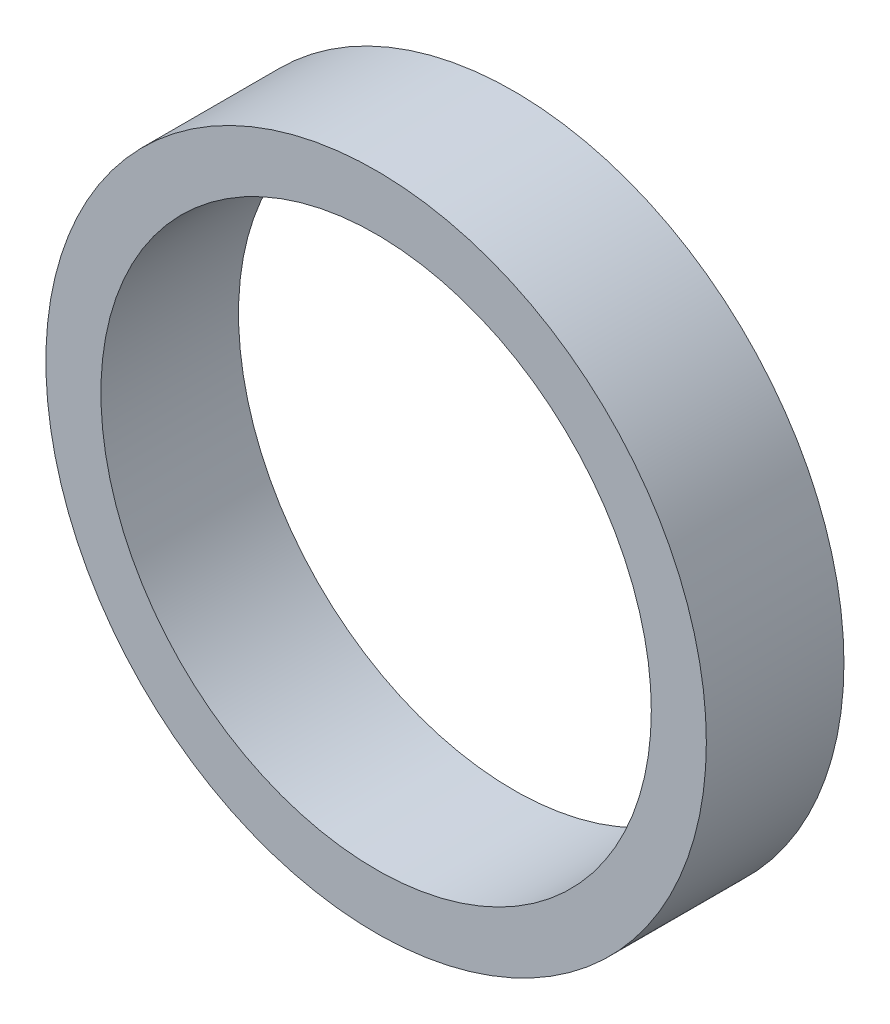
SolidWorks part; units mm, degrees
ref_plane "前视基准面" through (0, 0, 0) normal (0, 0, 1) x (1, 0, 0)
ref_plane "上视基准面" through (0, 0, 0) normal (0, 1, 0) x (1, 0, 0)
ref_plane "右视基准面" through (0, 0, 0) normal (1, 0, 0) x (0, 0, -1)
sketch "草图2" plane through (0, 0, 0) normal (0, 0, 1) x (1, 0, 0)
  circle A0 centre (0, 0) radius 20
  circle A1 centre (0, 0) radius 24
extrude "凸台-拉伸1" add sketch "草图2" along normal blind 10
